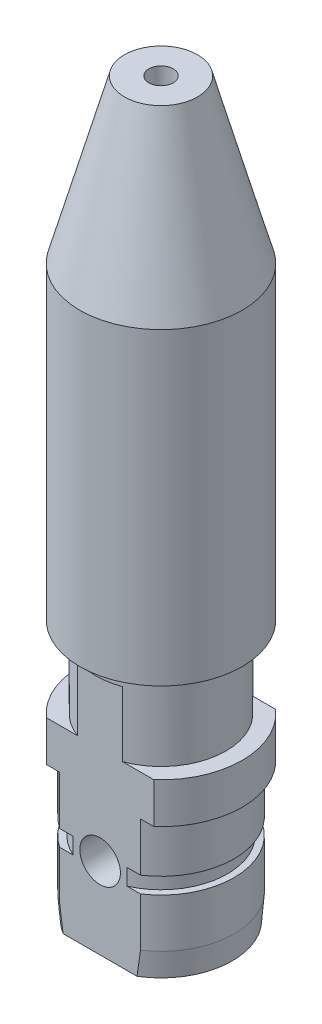
SolidWorks part; units mm, degrees
ref_plane "Front Plane" through (0, 0, 0) normal (0, 0, 1) x (1, 0, 0)
ref_plane "Top Plane" through (0, 0, 0) normal (0, 1, 0) x (1, 0, 0)
ref_plane "Right Plane" through (0, 0, 0) normal (1, 0, 0) x (0, 0, -1)
sketch "Sketch1" plane through (0, 0, 0) normal (0, 0, 1) x (1, 0, 0)
  line L0 (0, 0) -> (0, 9.7362) construction
  line L1 (-1.5, -45.8543) -> (-1.5, 44.1457)
  line L2 (-1.5, 44.1457) -> (-4.5, 44.1457)
  line L3 (-4.5, 44.1457) -> (-10, 24.1457)
  line L4 (-10, 24.1457) -> (-10, -13.8543)
  line L5 (-10, -28.8543) -> (-9, -28.8543)
  line L6 (-9, -28.8543) -> (-9, -34.8543)
  line L7 (-9, -34.8543) -> (-8.2, -34.8543)
  line L8 (-8.2, -34.8543) -> (-8.2, -36.8543)
  line L9 (-9, -36.8543) -> (-8.2, -36.8543)
  line L10 (-9, -36.8543) -> (-9, -42.8543)
  line L11 (-9, -42.8543) -> (-8.7723, -45.8543)
  line L12 (-8.7723, -45.8543) -> (-1.5, -45.8543)
  line L13 (-10, -23.8543) -> (-8, -23.8543)
  line L14 (-8, -23.8543) -> (-8, -13.8543)
  line L15 (-8, -13.8543) -> (-10, -13.8543)
  line L16 (-10, -23.8543) -> (-10, -28.8543)
  dimension "D1" = 3
  dimension "D2" = 20
  dimension "D3" = 3
  dimension "D4" = 20
  dimension "D5" = 90
  dimension "D6" = 3
  dimension "D7" = 6
  dimension "D8" = 2
  dimension "D9" = 0.8
  dimension "D10" = 6
  dimension "D11" = 1
  dimension "D12" = 0.8
  dimension "D13" = 10
  dimension "D14" = 5
  dimension "D15" = 2
revolve "Revolve1" add sketch "Sketch1" angle 360 about L0
sketch "Sketch2" plane through (0, -45.8543, 0) normal (0, -1, 0) x (-1, 0, 0)
  line L1 (13.1551, -7.5) -> (-13.1551, -7.5)
  line L2 (13.1551, -7.5) -> (13.1551, 7.5)
  line L3 (13.1551, 7.5) -> (-13.1551, 7.5)
  line L4 (-13.1551, -7.5) -> (-13.1551, 7.5)
  line L5 (13.1551, -7.5) -> (-13.1551, 7.5) construction
  line L6 (13.1551, 7.5) -> (-13.1551, -7.5) construction
  point P0 (0, 0)
  dimension "D1" = 15
extrude "Cut-Extrude1" cut sketch "Sketch2" against normal blind 30 flip side to cut
sketch "Sketch3" plane through (0, 0, 7.5) normal (0, 0, 1) x (1, 0, 0)
  line L0 (4.5502, -45.8543) -> (-4.5502, -45.8543) construction
  circle A0 centre (0, -35.8543) radius 2.5
  dimension "D1" = 5
  dimension "D2" = 10
extrude "Cut-Extrude2" cut sketch "Sketch3" against normal blind 5
sketch "Sketch5" plane through (0, 0, -7.5) normal (0, 0, -1) x (-1, 0, 0)
  line L0 (4.5502, -45.8543) -> (-4.5502, -45.8543) construction
  circle A0 centre (0, -35.8543) radius 2.5
  dimension "D1" = 10
  dimension "D2" = 5
extrude "Cut-Extrude3" cut sketch "Sketch5" against normal blind 5
